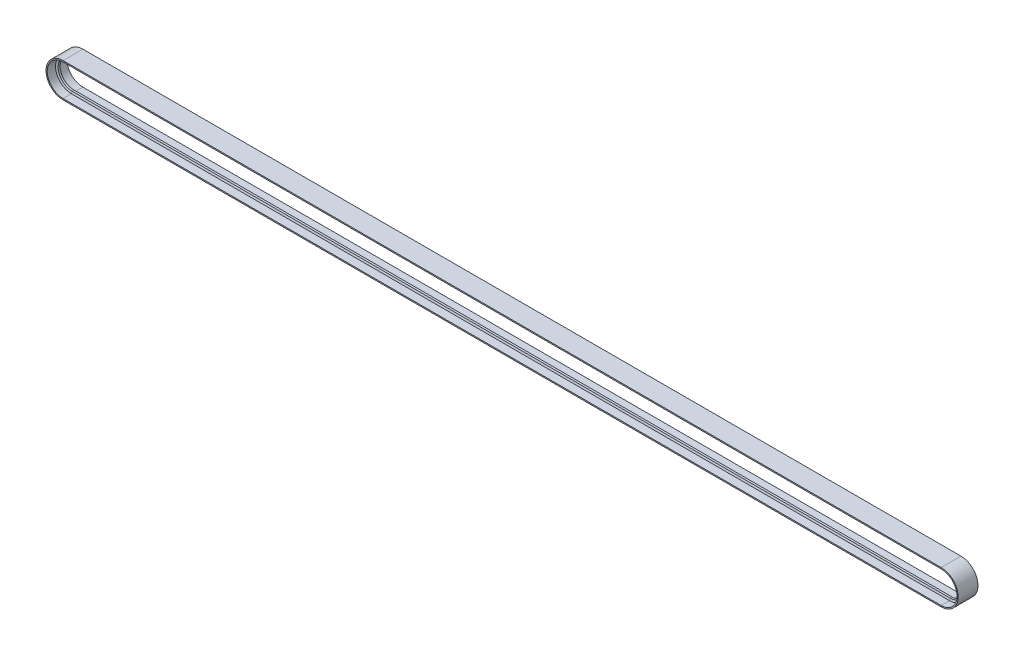
from build123d import *

# Parameters (mm, degrees)
EXTRUDE_1_DEPTH = 25


with BuildPart() as part:
    # 草图1 → 拉伸-薄壁1 (new, symmetric)
    with BuildSketch(Plane.XY):
        with BuildLine():
            Line((1108.5, -43), (-1108.5, -43))
            ThreePointArc((-1108.5, -43), (-1151.5, 0), (-1108.5, 43))
            Line((-1108.5, 43), (1108.5, 43))
            ThreePointArc((1108.5, 43), (1151.5, 0), (1108.5, -43))
        make_face()
        with BuildLine():
            Line((1108.5, -40), (-1108.5, -40))
            ThreePointArc((-1108.5, -40), (-1148.5, 0), (-1108.5, 40))
            Line((-1108.5, 40), (1108.5, 40))
            ThreePointArc((1108.5, 40), (1148.5, 0), (1108.5, -40))
        make_face(mode=Mode.SUBTRACT)
    extrude(amount=EXTRUDE_1_DEPTH, both=True)


with BuildPart() as body_2:
    # 扫描1: sweep along a path in 草图2
    with BuildLine(Plane.XY) as sweep_1_path:
        Line((-1108.5, -40), (1108.5, -40))
        ThreePointArc((1108.5, -40), (1148.5, 0), (1108.5, 40))
        Line((1108.5, 40), (-1108.5, 40))
        ThreePointArc((-1108.5, 40), (-1148.5, 0), (-1108.5, -40))
    # 草图3 → 扫描1 (sweep)
    with BuildSketch(Plane(origin=(0, 0, 0), x_dir=(0, 0, -1), z_dir=(1, 0, 0))):
        Polygon((4, 40), (-4, 40), (-2.5, 35), (2.5, 35), align=None)
    sweep(path=sweep_1_path.line)


solid = Compound([part.part, body_2.part])
